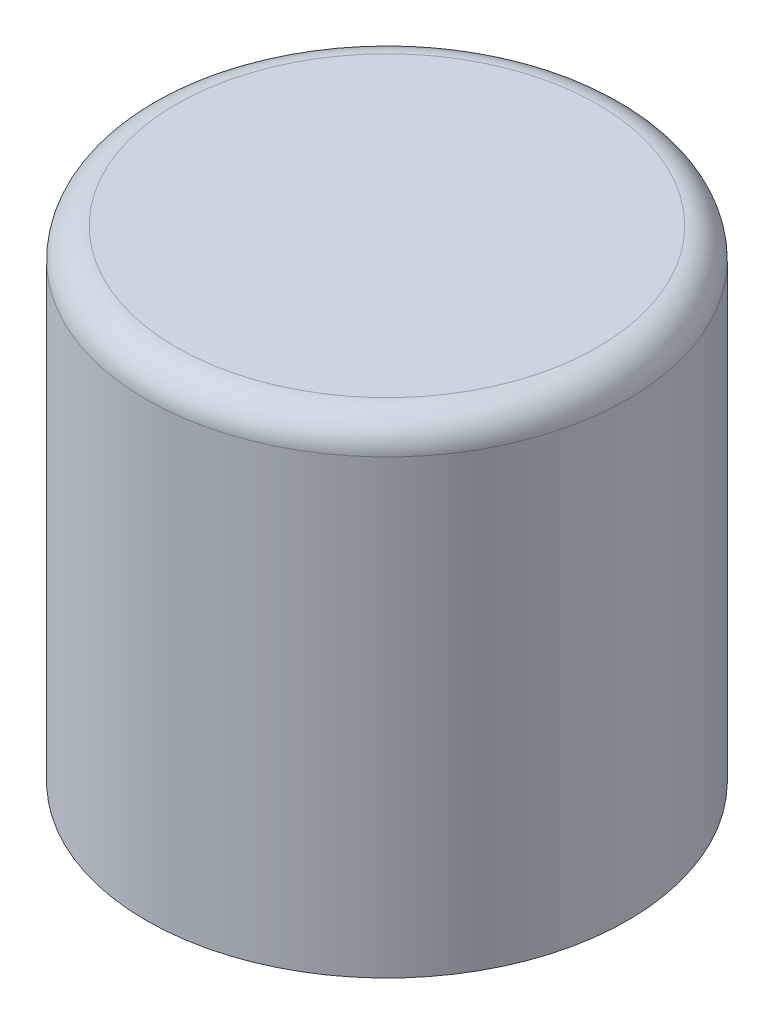
from build123d import *

# Parameters (mm, degrees)
SKETCH1_R           = 40
BOSS_EXTRUDE1_DEPTH = 80
FILLET1_R           = 5


with BuildPart() as part:
    # Sketch1 → Boss-Extrude1 (new body)
    with BuildSketch(Plane(origin=(0, 0, 0), x_dir=(1, 0, 0), z_dir=(0, 1, 0))):
        with Locations(Location((0, 0, 0), (0, 0, 270))):
            Circle(SKETCH1_R)
    extrude(amount=BOSS_EXTRUDE1_DEPTH)

    # Fillet1
    fillet1_edges = [part.edges().sort_by_distance(p)[0] for p in [
        (0, 80, -40),
    ]]
    fillet(fillet1_edges, radius=FILLET1_R)


solid = part.part
